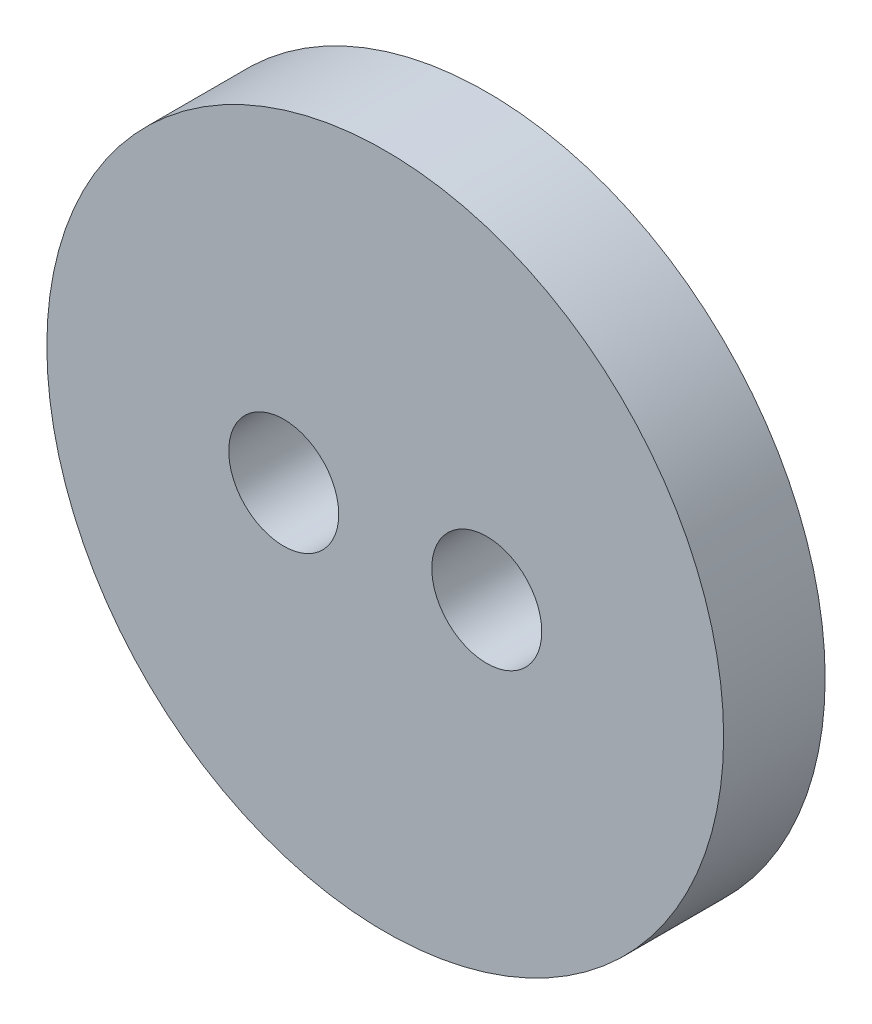
SolidWorks part; units mm, degrees
ref_plane "前视基准面" through (0, 0, 0) normal (0, 0, 1) x (1, 0, 0)
ref_plane "上视基准面" through (0, 0, 0) normal (0, 1, 0) x (1, 0, 0)
ref_plane "右视基准面" through (0, 0, 0) normal (1, 0, 0) x (0, 0, -1)
sketch "草图1" plane through (0, 0, 0) normal (0, 0, 1) x (1, 0, 0)
  circle A0 centre (0, 0) radius 20
  circle A1 centre (6, 0) radius 3.25
  circle A2 centre (-6, 0) radius 3.25
  dimension "D1" = 40
  dimension "D2" = 6.5
  dimension "D3" = 6.5
  dimension "D5" = 6
  dimension "D4" = 6
extrude "凸台-拉伸1" add sketch "草图1" along normal blind 6
